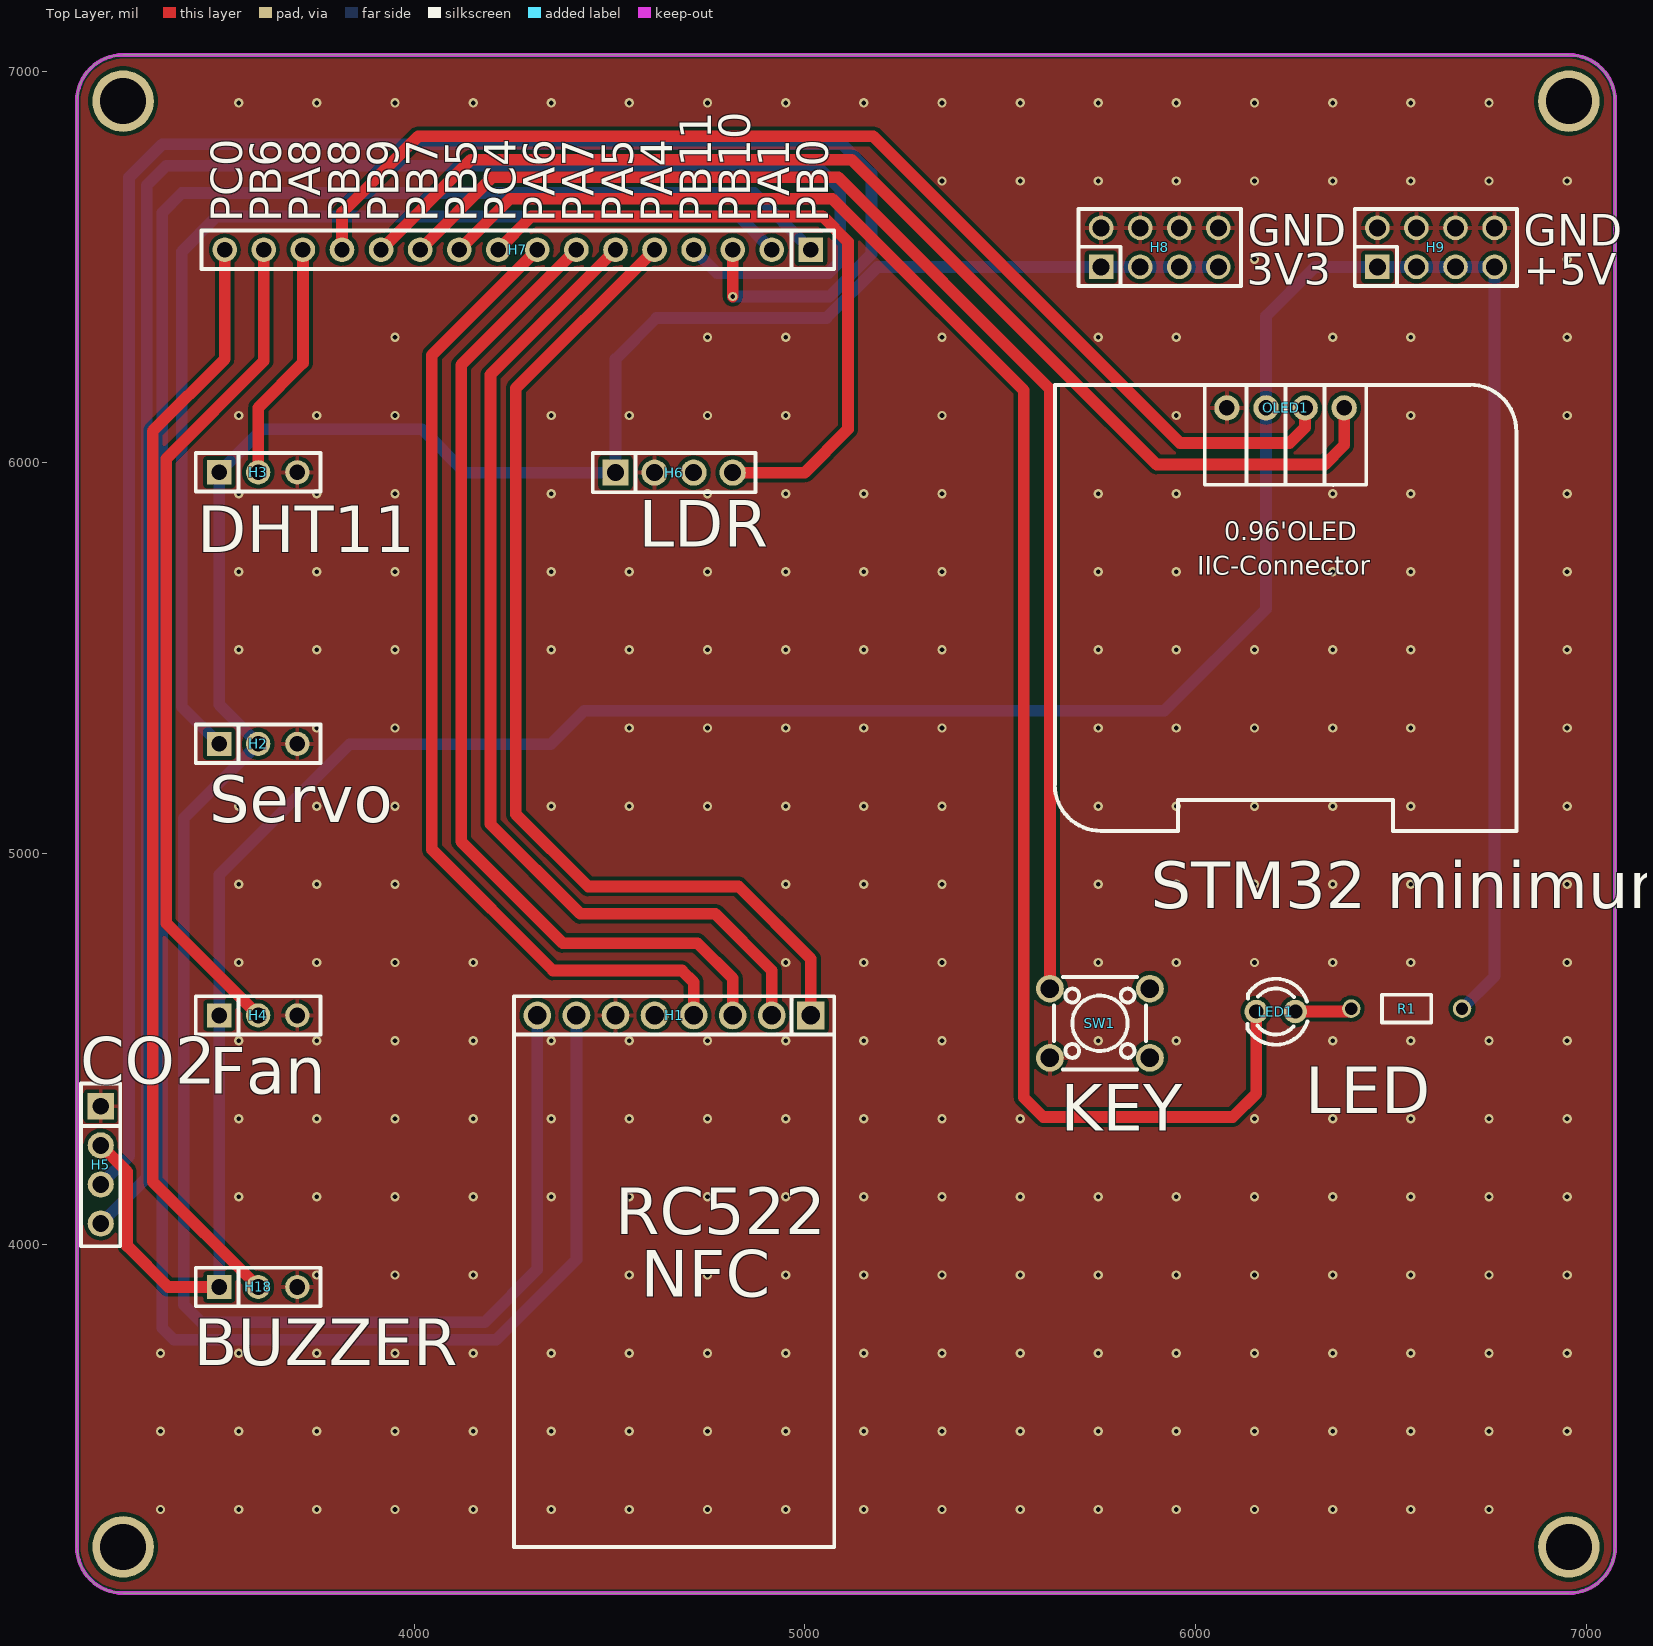
[diagram p0: Top Layer view]
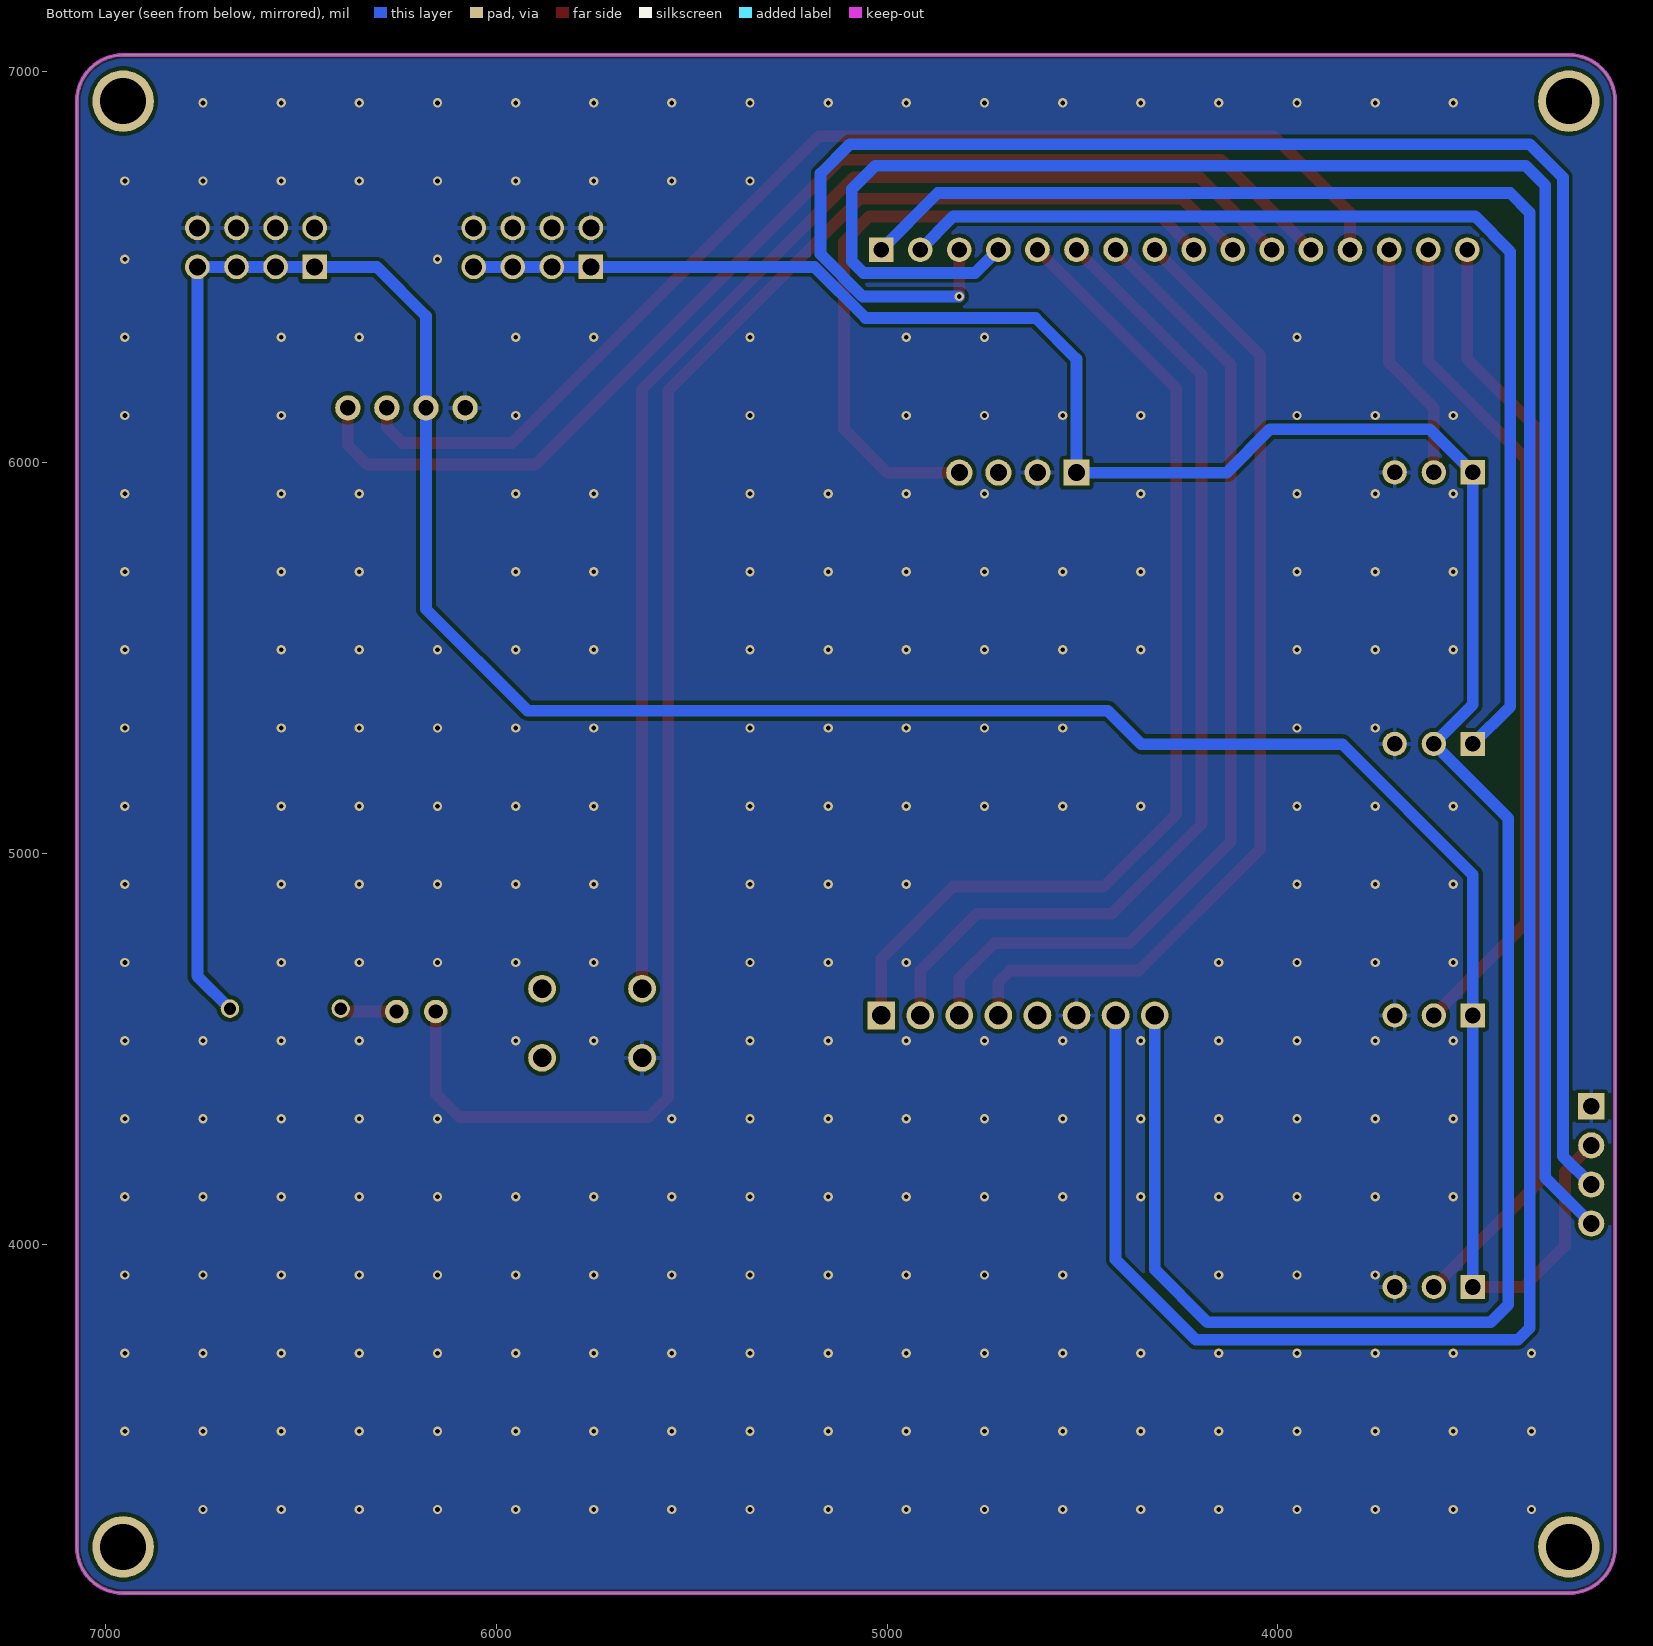
[diagram p1: Bottom Layer view, seen from below]
# Altium PCB MISC52124.pcbdoc
Units mil, origin at the board's own origin, x right, y up, seen from the top; angles counter-clockwise.
Board outline 3937.01 x 3937.01 mil, 2 copper layers (Top Layer, Bottom Layer), stack 62.206 mil thick; 14 components, 20 nets, 76 pads, 266 vias.

## Layer stack, top to bottom
Top Solder Mask Layer: solder mask 0.394, Dk 3.3
Top Layer: signal copper 1.379
Dielectric1: surface 59.449, FR4, Dk 4.5
Bottom Layer: signal copper 1.378
Bottom Solder Mask Layer: solder mask 0.394, Dk 3.3

## Board outline
3254.61,7043.5 ccw(c3254.61,6925.39) 3136.5,6925.39 3136.5,3224.61 ccw(c3254.61,3224.61) 3254.61,3106.5 6955.39,3106.5 ccw(c6955.39,3224.61) 7073.5,3224.61 7073.5,6925.39 ccw(c6955.39,6925.39) 6955.39,7043.5 3254.61,7043.5

## Design rules (kind name [scope] priority, off if disabled: settings)
BoardOutlineClearance copperThickness2oz_1 [All] p2 off: genericclearance=7.99 ignorepadtopadclearanceinfootprint=FALSE except(0: Arc-SplitContinuation Track-SplitContinuation SMDPad-SplitContinuation THPad-SplitContinuation Via-SplitContinuation Fill-SplitContinuation Region-SplitContinuation Poly-SplitContinuation Text-SplitContinuation Hole-SplitContinuation; 5.98: Arc-CutoutEdge Track-CutoutEdge SMDPad-CutoutEdge THPad-CutoutEdge Via-CutoutEdge Text-CutoutEdge; 6.9: Hole-OutlineEdge Hole-CutoutEdge; 10: Poly-OutlineEdge Poly-CutoutEdge; 11.81: Arc-OutlineEdge Track-OutlineEdge SMDPad-OutlineEdge THPad-OutlineEdge Via-OutlineEdge Fill-OutlineEdge Region-OutlineEdge Text-OutlineEdge Fill-CutoutEdge Region-CutoutEdge)
BoardOutlineClearance Plane_innerPlane_1 [All] p4 off: genericclearance=4.02 ignorepadtopadclearanceinfootprint=FALSE except(0: Arc-SplitContinuation Track-SplitContinuation SMDPad-SplitContinuation THPad-SplitContinuation Via-SplitContinuation Fill-SplitContinuation Region-SplitContinuation Poly-SplitContinuation Text-SplitContinuation Hole-SplitContinuation; 5.98: Arc-CutoutEdge Track-CutoutEdge SMDPad-CutoutEdge THPad-CutoutEdge Via-CutoutEdge Text-CutoutEdge; 6.9: Hole-OutlineEdge Hole-CutoutEdge; 10: Poly-OutlineEdge Poly-CutoutEdge; 11.81: Arc-OutlineEdge Track-OutlineEdge SMDPad-OutlineEdge THPad-OutlineEdge Via-OutlineEdge Fill-OutlineEdge Region-OutlineEdge Text-OutlineEdge Fill-CutoutEdge Region-CutoutEdge)
BoardOutlineClearance Copper_copperRegion_1 [All] p6 off: genericclearance=4.02 ignorepadtopadclearanceinfootprint=FALSE except(0: Arc-SplitContinuation Track-SplitContinuation SMDPad-SplitContinuation THPad-SplitContinuation Via-SplitContinuation Fill-SplitContinuation Region-SplitContinuation Poly-SplitContinuation Text-SplitContinuation Hole-SplitContinuation; 5.98: Arc-CutoutEdge Track-CutoutEdge SMDPad-CutoutEdge THPad-CutoutEdge Via-CutoutEdge Text-CutoutEdge; 6.9: Hole-OutlineEdge Hole-CutoutEdge; 10: Poly-OutlineEdge Poly-CutoutEdge; 11.81: Arc-OutlineEdge Track-OutlineEdge SMDPad-OutlineEdge THPad-OutlineEdge Via-OutlineEdge Fill-OutlineEdge Region-OutlineEdge Text-OutlineEdge Fill-CutoutEdge Region-CutoutEdge)
BoardOutlineClearance copperThickness1oz_1 [All] p8: genericclearance=4.02 ignorepadtopadclearanceinfootprint=FALSE except(0: Arc-SplitContinuation Track-SplitContinuation SMDPad-SplitContinuation THPad-SplitContinuation Via-SplitContinuation Fill-SplitContinuation Region-SplitContinuation Poly-SplitContinuation Text-SplitContinuation Hole-SplitContinuation; 5.98: Arc-CutoutEdge Track-CutoutEdge SMDPad-CutoutEdge THPad-CutoutEdge Via-CutoutEdge Text-CutoutEdge; 6.9: Hole-OutlineEdge Hole-CutoutEdge; 10: Poly-OutlineEdge Poly-CutoutEdge; 11.81: Arc-OutlineEdge Track-OutlineEdge SMDPad-OutlineEdge THPad-OutlineEdge Via-OutlineEdge Fill-OutlineEdge Region-OutlineEdge Text-OutlineEdge Fill-CutoutEdge Region-CutoutEdge)
Clearance copperThickness2oz [All] p1 off: gap=7.99 ignorepadtopadclearanceinfootprint=FALSE except(5.98: SMDPad-Track SMDPad-SMDPad THPad-Track SMDPad-THPad THPad-THPad Track-Via SMDPad-Via THPad-Via Via-Via Fill-SMDPad Region-SMDPad Fill-THPad Region-THPad Fill-Via Region-Via Fill-Fill Fill-Region Region-Region Arc-Track Arc-SMDPad Arc-THPad Arc-Via Fill-Arc Region-Arc Arc-Arc Text-Track SMDPad-Text Text-THPad Text-Via Fill-Text Region-Text Arc-Text Text-Text; 6.9: Hole-Track Hole-SMDPad Hole-THPad Hole-Via Fill-Hole Region-Hole Hole-Arc Hole-Text; 10: Poly-Track Poly-SMDPad Poly-THPad Poly-Via Poly-Fill Poly-Region Poly-Poly Poly-Arc Poly-Text Poly-Hole; 11.81: Fill-Track Region-Track)
Clearance Plane_innerPlane [All] p3 off: gap=4.02 ignorepadtopadclearanceinfootprint=FALSE except(5.98: SMDPad-Track SMDPad-SMDPad THPad-Track SMDPad-THPad THPad-THPad Track-Via SMDPad-Via THPad-Via Via-Via Fill-SMDPad Region-SMDPad Fill-THPad Region-THPad Fill-Via Region-Via Fill-Fill Fill-Region Region-Region Arc-Track Arc-SMDPad Arc-THPad Arc-Via Fill-Arc Region-Arc Arc-Arc Text-Track SMDPad-Text Text-THPad Text-Via Fill-Text Region-Text Arc-Text Text-Text; 6.9: Hole-Track Hole-SMDPad Hole-THPad Hole-Via Fill-Hole Region-Hole Hole-Arc Hole-Text; 10: Poly-Track Poly-SMDPad Poly-THPad Poly-Via Poly-Fill Poly-Region Poly-Poly Poly-Arc Poly-Text Poly-Hole; 11.81: Fill-Track Region-Track)
Clearance Copper_copperRegion [All] p5 off: gap=4.02 ignorepadtopadclearanceinfootprint=FALSE except(5.98: SMDPad-Track SMDPad-SMDPad THPad-Track SMDPad-THPad THPad-THPad Track-Via SMDPad-Via THPad-Via Via-Via Fill-SMDPad Region-SMDPad Fill-THPad Region-THPad Fill-Via Region-Via Fill-Fill Fill-Region Region-Region Arc-Track Arc-SMDPad Arc-THPad Arc-Via Fill-Arc Region-Arc Arc-Arc Text-Track SMDPad-Text Text-THPad Text-Via Fill-Text Region-Text Arc-Text Text-Text; 6.9: Hole-Track Hole-SMDPad Hole-THPad Hole-Via Fill-Hole Region-Hole Hole-Arc Hole-Text; 10: Poly-Track Poly-SMDPad Poly-THPad Poly-Via Poly-Fill Poly-Region Poly-Poly Poly-Arc Poly-Text Poly-Hole; 11.81: Fill-Track Region-Track)
Clearance copperThickness1oz [All] p7: gap=4.02 ignorepadtopadclearanceinfootprint=FALSE except(5.98: SMDPad-Track SMDPad-SMDPad THPad-Track SMDPad-THPad THPad-THPad Track-Via SMDPad-Via THPad-Via Via-Via Fill-SMDPad Region-SMDPad Fill-THPad Region-THPad Fill-Via Region-Via Fill-Fill Fill-Region Region-Region Arc-Track Arc-SMDPad Arc-THPad Arc-Via Fill-Arc Region-Arc Arc-Arc Text-Track SMDPad-Text Text-THPad Text-Via Fill-Text Region-Text Arc-Text Text-Text; 6.9: Hole-Track Hole-SMDPad Hole-THPad Hole-Via Fill-Hole Region-Hole Hole-Arc Hole-Text; 10: Poly-Track Poly-SMDPad Poly-THPad Poly-Via Poly-Fill Poly-Region Poly-Poly Poly-Arc Poly-Text Poly-Hole; 11.81: Fill-Track Region-Track)
DiffPairsRouting differentialPair [All] p1: maxlimit=6 minlimit=6 mostfreqgap=6 toplayer_minwidth=5 toplayer_prefwidth=10 toplayer_maxwidth=100 toplayer_mingap=6 toplayer_prefgap=6 toplayer_maxgap=6 bottomlayer_minwidth=5 bottomlayer_prefwidth=10 bottomlayer_maxwidth=100 bottomlayer_mingap=6 bottomlayer_prefgap=6 bottomlayer_maxgap=6 maxuncoupledlength=10
HoleToHoleClearance otherClearance [All] p1: gap=11.81 allowstackedmicrovias=TRUE
Length netLength [All] p1: minlimit=0 maxlimit=0
PasteMaskExpansion pasteMaskExpansion [All] p1: expansion=0
PlaneConnect innerPlane [All] p1: planeconnectstyle=Relief reliefexpansion=20 reliefentries=4 reliefconductorwidth=10 reliefairgap=10
PolygonConnect copperRegion [All] p1: connectstyle=Relief reliefconductorwidth=10 reliefentries=4 polygonreliefangle="90 Angle" airgapwidth=10 via.connectstyle=Relief via.reliefconductorwidth=10 via.reliefentries=4 via.polygonreliefangle="90 Angle" via.airgapwidth=10
RoutingVias viaSize [All] p1: holewidth=12.01 width=24.02 viastyle="Through Hole" minholewidth=11.81 minwidth=19.68 maxholewidth=248.03 maxwidth=393.7
SolderMaskExpansion solderMaskExpansion [IsVia] p1: expansion=-1000 istentingtop=TRUE
SolderMaskExpansion solderMaskExpansion [All] p2: expansion=2 istentingtop=FALSE
Width copperThickness2oz_2 [All] p1 off: maxlimit=100 minlimit=8 preferedwidth=10
Width copperThickness1oz_2 [All] p2: maxlimit=100 minlimit=5 preferedwidth=10

## Components (designator, comment, footprint, x,y, rotation, side; value= is the part's Value field where it differs from the comment)
H1 "" HDR-TH_8P-P2.54-V-F-1 4665,4585 r180 top
H2 "" HDR-TH_3P-P2.54-V-F 3600.6,5280 r0 top
H3 "" HDR-TH_3P-P2.54-V-F 3600.6,5975 r0 top
H4 "" HDR-TH_3P-P2.54-V-F 3600.6,4585 r0 top
H5 "" HDR-TH_4P-P2.54-V-F 3197.5,4202.5 r270 top
H6 "" HDR-TH_4P-P2.54-V-F 4665,5974.21 r0 top
H7 "" HDR-TH_16P-P2.54-V-F 4265,6545 r180 top
H8 "" HDR-TH_8P-P2.54-V-F-R2-C4-S2.54-1 5908,6550.79 r0 top
H9 "" HDR-TH_8P-P2.54-V-F-R2-C4-S2.54-1 6615,6550.79 r0 top
H18 "" HDR-TH_3P-P2.54-V-F 3600.6,3890 r0 top
LED1 "" LED_TH-3mm 6205,4595 r180 top
OLED1 "" 0.96OLED_4P 6230,6140 r0 top
R1 "300" Res_1/8W 6540,4600 r0 top
SW1 "" SW-TH_4P-L6.0-W6.0-P4.50-LS6.5 5755,4565 r0 top

## Footprints (in the part's own frame and the unit in brackets; to place one, negate y for a bottom-side part, rotate by r counter-clockwise, add the part's x,y. Pads: shape width x height; smd on the part's side, far side on the other; paste and mask are expansions set on the pad)
0.96OLED_4P [mm]
  round 1.65 hole 1 copper offset 0,0: 1(-3.81,-0.001) 2(-1.27,0.002) 3(1.27,0.002) 4(3.81,0.002)
  silkscreen extent -15,-27.5 15,1.5
HDR-TH_3P-P2.54-V-F [mil]
  rect 62x62 hole 40.16: 1(-100,0)
  round 62 hole 40.16: 2(0,0) 3(100,0)
  silkscreen extent -160,-49 160,49
HDR-TH_4P-P2.54-V-F [mm]
  rect 1.7x1.7 hole 1.1: 1(-3.81,0)
  round 1.7 hole 1.1: 2(-1.27,0) 3(1.27,0) 4(3.81,0)
  silkscreen extent -5.29,-1.27 5.29,1.27
HDR-TH_8P-P2.54-V-F-1 [mm]
  rect 1.8x1.8 hole 1.2: 1(-8.89,0)
  round 1.8 hole 1.2: 2(-6.35,0) 3(-3.81,0) 4(-1.27,0) 5(1.27,0) 6(3.81,0) 7(6.35,0) 8(8.89,0)
  silkscreen extent -10.41,-1.25 10.41,1.25
HDR-TH_8P-P2.54-V-F-R2-C4-S2.54-1 [mm]
  rect 1.6x1.6 hole 1.1: 1(-3.81,-1.27)
  round 1.6 hole 1.1: 2(-3.81,1.27) 3(-1.27,-1.27) 4(-1.27,1.27) 5(1.27,-1.27) 6(1.27,1.27) 7(3.81,-1.27) 8(3.81,1.27)
  silkscreen extent -5.28,-2.5 5.28,2.5
HDR-TH_16P-P2.54-V-F [mm]
  rect 1.6x1.6 hole 1: 1(-19.05,0)
  round 1.6 hole 1: 2(-16.51,0) 3(-13.97,0) 4(-11.43,0) 5(-8.89,0) 6(-6.35,0) 7(-3.81,0) 8(-1.27,0) 9(1.27,0) 10(3.81,0) 11(6.35,0) 12(8.89,0) 13(11.43,0) 14(13.97,0) 15(16.51,0) 16(19.05,0)
  silkscreen extent -20.57,-1.25 20.57,1.25
LED_TH-3mm [mil]
  round 60 hole 36 paste+0 mask+2: 1(-50,0) 2(50,0)
  silkscreen extent -81,-84 72,85
Res_1/8W [mil]
  round 47.2 hole 31.5 paste+0 mask+2: 1(-141.7,2.48) 2(141.7,2.48)
  silkscreen extent -63,-33 63,38
SW-TH_4P-L6.0-W6.0-P4.50-LS6.5 [mm]
  round 1.8 hole 1.2: 1(-3.25,2.25) 2(3.25,2.25) 3(-3.25,-2.25) 4(3.25,-2.25)
  silkscreen extent -3,-3 3,3

## Free pads (board coordinates)
  round 157.48 hole 118.11: 1(3254.61,6925.39) 1(3254.61,3224.61) 1(6955.39,6925.39) 1(6955.39,3224.61)

## Via types
v1: diameter 24.02, hole 12, Top Layer to Bottom Layer, 266 vias

## Nets (pads, with @x,y where several pads share a name; then routed paths per layer and width w, separated by ;. In a path a pad name is that pad's centre, name@x,y a point inside that pad or via, vN(x,y) a via of type N, cw(c..) or ccw(c..) an arc to the next point about the centre after c; other vN are vias at no path point)
$1N16986: LED1.1 R1.1 | length 146.4
  Top Layer w30: LED1.1 6390.82,4595 R1.1
+5V: H4.1 H5.2 H9.1 H9.3 H9.5 H9.7 H18.1 OLED1.2 R1.2 | length 7900.9
  Top Layer w30: H5.2 3265,4185 3265,3995 3370,3890 H18.1
  Bottom Layer w30: H18.1 H4.1 3500.6,4945.6 3834.21,5279.21 4349.21,5279.21 4435,5365 5920,5365 6180,5625 6180,6140.05 6180,6375 6305.79,6500.79 H9.1 H9.3 H9.5 H9.7 6765,4685.78 R1.2
GND: H1.6 H2.3 H3.3 H4.3 H5.1 H6.2 H8.2 H8.4 H8.6 H8.8 H9.2 H9.4 H9.6 H9.8 H18.3 OLED1.1 SW1.3
  other v1: 3350.6,3320.6 3550.6,3320.6 3750.6,3320.6 3950.6,3320.6 4150.6,3320.6 4350.6,3320.6 4550.6,3320.6 4750.6,3320.6 4950.6,3320.6 5150.6,3320.6 5350.6,3320.6 5550.6,3320.6 5750.6,3320.6 5950.6,3320.6 6150.6,3320.6 6350.6,3320.6 6550.6,3320.6 6750.6,3320.6 3350.6,3520.6 3550.6,3520.6 3750.6,3520.6 3950.6,3520.6 4150.6,3520.6 4350.6,3520.6 4550.6,3520.6 4750.6,3520.6 4950.6,3520.6 5150.6,3520.6 5350.6,3520.6 5550.6,3520.6 5750.6,3520.6 5950.6,3520.6 6150.6,3520.6 6350.6,3520.6 6550.6,3520.6 6750.6,3520.6 6950.6,3520.6 3350.6,3720.6 3550.6,3720.6 3750.6,3720.6 3950.6,3720.6 4150.6,3720.6 4350.6,3720.6 4550.6,3720.6 4750.6,3720.6 4950.6,3720.6 5150.6,3720.6 5350.6,3720.6 5550.6,3720.6 5750.6,3720.6 5950.6,3720.6 6150.6,3720.6 6350.6,3720.6 6550.6,3720.6 6750.6,3720.6 6950.6,3720.6 3750.6,3920.6 3950.6,3920.6 4150.6,3920.6 4550.6,3920.6 4750.6,3920.6 4950.6,3920.6 5150.6,3920.6 5350.6,3920.6 5550.6,3920.6 5750.6,3920.6 5950.6,3920.6 6150.6,3920.6 6350.6,3920.6 6550.6,3920.6 6750.6,3920.6 6950.6,3920.6 3550.6,4120.6 3750.6,4120.6 3950.6,4120.6 4150.6,4120.6 4350.6,4120.6 4550.6,4120.6 4750.6,4120.6 4950.6,4120.6 5150.6,4120.6 5350.6,4120.6 5550.6,4120.6 5750.6,4120.6 5950.6,4120.6 6150.6,4120.6 6350.6,4120.6 6550.6,4120.6 6750.6,4120.6 6950.6,4120.6 3550.6,4320.6 3750.6,4320.6 3950.6,4320.6 4150.6,4320.6 4350.6,4320.6 4550.6,4320.6 4750.6,4320.6 4950.6,4320.6 5150.6,4320.6 5350.6,4320.6 5550.6,4320.6 6150.6,4320.6 6350.6,4320.6 6550.6,4320.6 6750.6,4320.6 6950.6,4320.6 3550.6,4520.6 3750.6,4520.6 3950.6,4520.6 4150.6,4520.6 4350.6,4520.6 4550.6,4520.6 4750.6,4520.6 4950.6,4520.6 5150.6,4520.6 5350.6,4520.6 5750.6,4520.6 5950.6,4520.6 6350.6,4520.6 6550.6,4520.6 6750.6,4520.6 6950.6,4520.6 3550.6,4720.6 3750.6,4720.6 3950.6,4720.6 4150.6,4720.6 4950.6,4720.6 5150.6,4720.6 5350.6,4720.6 5750.6,4720.6 5950.6,4720.6 6150.6,4720.6 6350.6,4720.6 6550.6,4720.6 6950.6,4720.6 3550.6,4920.6 3750.6,4920.6 3950.6,4920.6 4950.6,4920.6 5150.6,4920.6 5350.6,4920.6 5750.6,4920.6 5950.6,4920.6 6150.6,4920.6 6350.6,4920.6 6550.6,4920.6 6950.6,4920.6 3550.6,5120.6 3750.6,5120.6 3950.6,5120.6 4350.6,5120.6 4550.6,5120.6 4750.6,5120.6 4950.6,5120.6 5150.6,5120.6 5350.6,5120.6 5750.6,5120.6 5950.6,5120.6 6150.6,5120.6 6350.6,5120.6 6550.6,5120.6 6950.6,5120.6 3750.6,5320.6 3950.6,5320.6 4550.6,5320.6 4750.6,5320.6 4950.6,5320.6 5150.6,5320.6 5350.6,5320.6 5750.6,5320.6 5950.6,5320.6 6150.6,5320.6 6350.6,5320.6 6550.6,5320.6 6950.6,5320.6 3550.6,5520.6 3750.6,5520.6 3950.6,5520.6 4350.6,5520.6 4550.6,5520.6 4750.6,5520.6 4950.6,5520.6 5150.6,5520.6 5350.6,5520.6 5750.6,5520.6 5950.6,5520.6 6150.6,5520.6 6350.6,5520.6 6550.6,5520.6 6950.6,5520.6 3550.6,5720.6 3750.6,5720.6 3950.6,5720.6 4350.6,5720.6 4550.6,5720.6 4750.6,5720.6 4950.6,5720.6 5150.6,5720.6 5350.6,5720.6 5750.6,5720.6 5950.6,5720.6 6350.6,5720.6 6550.6,5720.6 6950.6,5720.6 3550.6,5920.6 3750.6,5920.6 3950.6,5920.6 4350.6,5920.6 4750.6,5920.6 4950.6,5920.6 5150.6,5920.6 5350.6,5920.6 5750.6,5920.6 5950.6,5920.6 6350.6,5920.6 6550.6,5920.6 6950.6,5920.6 3550.6,6120.6 3750.6,6120.6 3950.6,6120.6 4350.6,6120.6 4550.6,6120.6 4750.6,6120.6 4950.6,6120.6 5350.6,6120.6 5950.6,6120.6 6550.6,6120.6 6950.6,6120.6 3950.6,6320.6 4750.6,6320.6 4950.6,6320.6 5350.6,6320.6 5750.6,6320.6 5950.6,6320.6 6350.6,6320.6 6550.6,6320.6 6950.6,6320.6 6150.6,6520.6 6950.6,6520.6 5350.6,6720.6 5550.6,6720.6 5750.6,6720.6 5950.6,6720.6 6150.6,6720.6 6350.6,6720.6 6550.6,6720.6 6750.6,6720.6 6950.6,6720.6 3550.6,6920.6 3750.6,6920.6 3950.6,6920.6 4150.6,6920.6 4350.6,6920.6 4550.6,6920.6 4750.6,6920.6 4950.6,6920.6 5150.6,6920.6 5350.6,6920.6 5550.6,6920.6 5750.6,6920.6 5950.6,6920.6 6150.6,6920.6 6350.6,6920.6 6550.6,6920.6 6750.6,6920.6
PA1: H2.1 H7.2 | length 2882.1
  Bottom Layer w30: H2.1 3405,5375.6 3405,6540 3495,6630 4830,6630 H7.2
PA4: H1.1 H7.5 | length 2645.3
  Top Layer w30: H7.5 4260,6190 4260,5100 4445,4915 4830,4915 5015,4730 H1.1
PA5: H1.2 H7.6 | length 2592.9
  Top Layer w30: H7.6 4195,6225 4195,5075 4425,4845 4770,4845 4915,4700 H1.2
PA6: H1.4 H7.8 | length 2542.7
  Top Layer w30: H7.8 4045,6275 4045,5010 4355,4700 4685,4700 4715,4670 H1.4
PA7: H1.3 H7.7 | length 2572.2
  Top Layer w30: H7.7 4120,6250 4120,5030 4380,4770 4725,4770 4815,4680 H1.3
PA8: H3.2 H7.14 | length 617.4
  Top Layer w30: H3.2 3600.6,6140.6 3715,6255 H7.14
PB0: H1.7 H7.1 | length 6378.1
  Bottom Layer w30: H1.7 4415,3960 4210,3755 3385,3755 3355,3785 3355,6640 3405,6690 4870,6690 H7.1
PB5: H7.10 LED1.2 | length 4362.4
  Top Layer w30: H7.10 4245,6675 5070,6675 5560,6185 5560,4375 5610,4325 6095,4325 6155,4385 LED1.2
PB6: H4.2 H7.15 | length 2161.1
  Top Layer w30: H4.2 3365,4820.6 3365,6010 3615,6260 H7.15
PB7: H7.11 SW1.1 | length 3447.6
  Top Layer w30: H7.11 4200,6730 5085,6730 5627.05,6187.95 SW1.1
PB8: H7.13 OLED1.3 | length 3032.5
  Top Layer w30: H7.13 3815,6640 4010,6835 5175,6835 5960,6050 6240,6050 6280,6090 OLED1.3@6280,6140.05
PB9: H7.12 OLED1.4 | length 2999.1
  Top Layer w30: H7.12 4145,6775 5120,6775 5900,5995 6330,5995 6380,6045 OLED1.4@6380,6140.05
PB10: H5.3 H7.3 | length 5300.5
  Top Layer w30: v1(4815,6425) H7.3
  Bottom Layer w30: H5.3 3270,4225 3270,6730 3355,6815 5095,6815 5170,6740 5170,6533.11 5061.89,6425 v1(4815,6425)
PB11: H5.4 H7.4 | length 5124
  Bottom Layer w30: H5.4 3315,4170 3315,6710 3365,6760 5030,6760 5090,6700 5090,6515 5060,6485 4775,6485 H7.4
PC0: H7.16 H18.2 | length 2842.9
  Top Layer w30: H7.16 3515,6265 3330.98,6080.98 3330.98,4159.62 H18.2
PC4: H6.4 H7.9 | length 1778
  Top Layer w30: H7.9 4300,6630 5045,6630 5110,6565 5110,6085 4999.21,5974.21 H6.4
VCC: H1.8 H2.2 H3.1 H6.1 H8.1 H8.3 H8.5 H8.7 | length 6917.2
  Bottom Layer w30: H1.8 4315,3935 4180,3800 3455,3800 3410,3845 3410,5089.4 H2.2 3500.6,5380 H3.1 3610.6,6085 4020,6085 4130.79,5974.21 H6.1 4515,6265 4620,6370 5055,6370 5185.79,6500.79 H8.1 H8.3 H8.5 H8.7
pads on no net: H1.5 H6.3 SW1.2 SW1.4

## Polygon pours and split planes (outlines as drawn)
GND on Bottom Layer (solid, remove dead copper, pour order 2): 3065,7165 3065,3000 7240,3000 7240,7165
GND on Top Layer (solid, remove dead copper, pour order 0): 3000,7130 3000,3060 7385,3060 7385,7130

## Keep-outs
Board Outline Layer:
  the board outline again, w10

## Silkscreen, mask and mechanical layers (free items; w line width, h text height)
Top Silkscreen Layer:
  lines w10: 4255.16,3225 4255.16,4634.21 5075,4634.21 5075,3225 4255.16,3225
  text "PC0" at 3560,6615.3 h80 r90
  text "PB6" at 3660,6615.3 h80 r90
  text "PA8" at 3760,6615.3 h80 r90
  text "PB8" at 3860,6615.3 h80 r90
  text "PB9" at 3960,6615.3 h80 r90
  text "PB7" at 4060,6615.3 h80 r90
  text "PB5" at 4160,6615.3 h80 r90
  text "PC4" at 4260,6615.3 h80 r90
  text "PA6" at 4360,6615.3 h80 r90
  text "PA7" at 4460,6615.3 h80 r90
  text "PA5" at 4560,6615.3 h80 r90
  text "PA4" at 4660,6615.3 h80 r90
  text "PB11" at 4760,6615.3 h80 r90
  text "PB10" at 4860,6615.3 h80 r90
  text "PA1" at 4960,6615.3 h80 r90
  text "PB0" at 5060,6615.3 h80 r90
  text "GND" at 6133.15,6555 h80
  text "GND" at 6839.16,6555 h80
  text "3V3" at 6130.95,6455 h80
  text "+5V" at 6839.16,6455 h80
  text "LDR" at 4575,5785 h120
  text "DHT11" at 3445,5770 h120
  text "Servo" at 3475,5080 h120
  text "STM32 minimum system" at 5885,4860 h120
  text "CO2" at 3145,4410 h120
  text "Fan" at 3475,4385 h120
  text "LED" at 6280,4335 h120
  text "KEY" at 5655,4290 h120
  text "RC522" at 4515,4025 h120
  text "NFC" at 4580,3865 h120
  text "BUZZER" at 3435,3690 h120